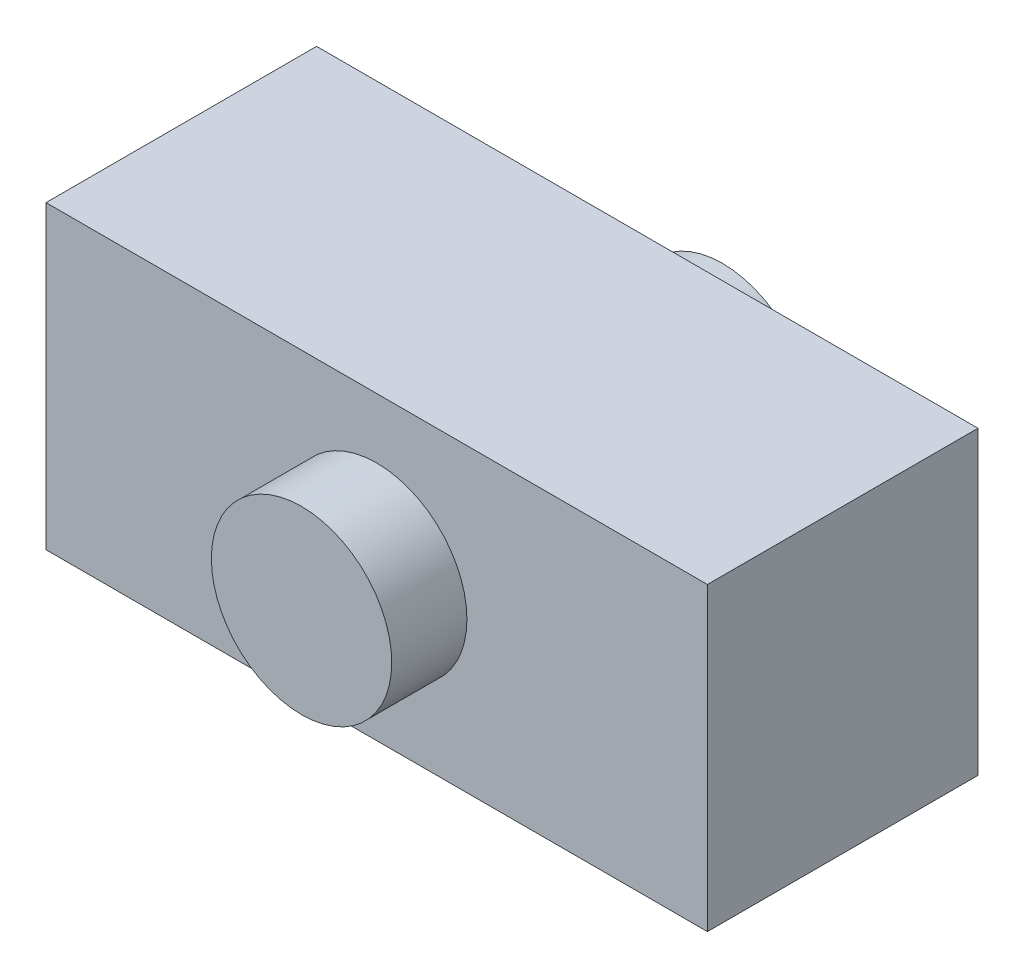
SolidWorks part; units mm, degrees
ref_plane "前视基准面" through (0, 0, 0) normal (0, 0, 1) x (1, 0, 0)
ref_plane "上视基准面" through (0, 0, 0) normal (0, 1, 0) x (1, 0, 0)
ref_plane "右视基准面" through (0, 0, 0) normal (1, 0, 0) x (0, 0, -1)
other "Configuration Table"
sketch "草图1" plane through (0, 0, 0) normal (0, 0, 1) x (1, 0, 0)
  line L0 (-22, -10) -> (22, -10)
  line L1 (22, -10) -> (22, 10)
  line L2 (22, 10) -> (-22, 10)
  line L3 (-22, 10) -> (-22, -10)
  point P0 (0, 0)
  dimension "D1" = 22
  dimension "D2" = 44
  dimension "D3" = 10
  dimension "D4" = 20
extrude "凸台-拉伸1" add sketch "草图1" against normal mid plane 18
sketch "草图2" plane through (0, 0, 0) normal (0, 0, 1) x (1, 0, 0)
  circle A0 centre (0, 0) radius 6
  point P0 (0, 0)
  dimension "D1" = 12
extrude "凸台-拉伸2" add sketch "草图2" against normal mid plane 28
